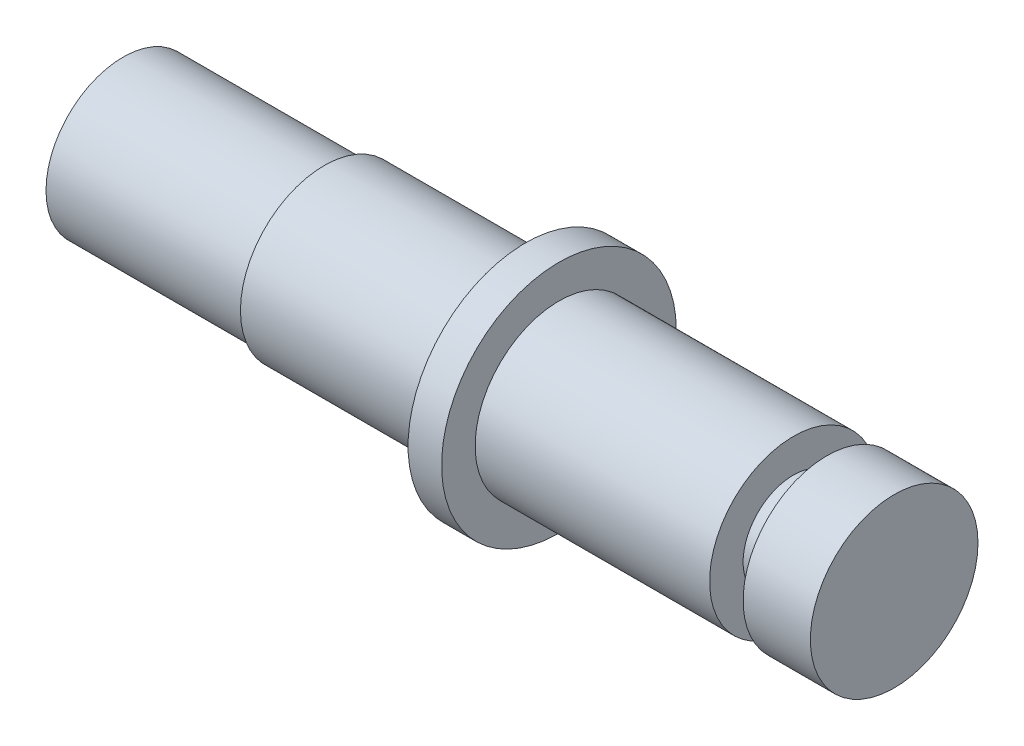
SolidWorks part; units mm, degrees
ref_plane "Front Plane" through (0, 0, 0) normal (0, 0, 1) x (1, 0, 0)
ref_plane "Top Plane" through (0, 0, 0) normal (0, 1, 0) x (1, 0, 0)
ref_plane "Right Plane" through (0, 0, 0) normal (1, 0, 0) x (0, 0, -1)
other "Configuration Table"
sketch "Sketch1" plane through (0, 0, 0) normal (1, 0, 0) x (0, 0, -1)
  circle A0 centre (0, 0) radius 2.3
extrude "Boss-Extrude1" add sketch "Sketch1" along normal blind 20
sketch "Sketch3" plane through (0, 0, 0) normal (0, 0, 1) x (1, 0, 0)
  line L0 (0, 2.3) -> (10, 2.3) construction
  line L1 (20, 2.3) -> (0, 2.3) construction
  line L2 (10, 2.3) -> (10, 2.5)
  line L3 (10, 2.5) -> (10.6945, 2.5)
  line L4 (10.6945, 2.5) -> (10.6945, 2.3)
  line L5 (10.6945, 2.3) -> (10, 2.3)
  line L6 (10, 2.3) -> (10, 0) construction
  line L7 (10, 0) -> (10.6945, 0)
revolve "Revolve1" add sketch "Sketch3" angle 360 about axis through (20, 0, 0) along (-1, 0, 0)
sketch "Sketch4" plane through (0, 0, 0) normal (-1, 0, 0) x (0, 0, 1)
  circle A0 centre (0, 0) radius 2.3
extrude "Boss-Extrude2" add sketch "Sketch4" along normal blind 2
sketch "Sketch5" plane through (20, 0, 0) normal (1, 0, 0) x (0, 0, -1)
  circle A0 centre (0, 0) radius 2.5
extrude "Boss-Extrude3" add sketch "Sketch5" against normal blind 10
sketch "Sketch6" plane through (0.9939, 0, 0) normal (0, 0, 1) x (1, 0, 0)
  line L0 (20, 2.5) -> (18, 2.5) construction
  line L2 (18, 2.5) -> (18, 1.4999)
  line L3 (18, 1.4999) -> (17, 1.4999)
  line L4 (17, 1.4999) -> (17, 2.5)
  line L5 (17, 2.5) -> (18, 2.5)
  line L6 (20, 0) -> (16.6857, 0) construction
revolve "Cut-Revolve1" cut sketch "Sketch6" angle 360 about L6
sketch "Sketch8" plane through (-2, 0, 0) normal (-1, 0, 0) x (0, 0, 1)
  line L0 (0, 0) -> (0, 2.3) construction
  circle A0 centre (0, 0) radius 2.3 construction
ref_plane "Plane1" through (0, 0, 0) normal (0, 0, 1) x (0, 1, 0)
sketch "Sketch9" plane through (0, 0, 0) normal (0, 0, 1) x (0, 1, 0)
  line L0 (1.5, 2) -> (2.3, -4.25) construction
  line L1 (0, 2) -> (2.3, 2) construction
  line L2 (2.3, -10) -> (2.3, 2) construction
  line L3 (2.3, -4.25) -> (0.75, -4.25)
  line L4 (0.75, -4.25) -> (0.75, -4.9347)
  line L5 (0.75, -4.9347) -> (2.3, -4.9347)
  line L6 (2.3, -4.9347) -> (2.3, -4.25)
  line L7 (0, 2) -> (0, -4.6531) construction
  line L8 (2.3, 2) -> (-2.3, 2) construction
  line L9 (-2.3, -4.25) -> (-0.75, -4.25)
  line L10 (-2.3, -4.9347) -> (-2.3, -4.25)
  line L11 (-0.75, -4.9347) -> (-2.3, -4.9347)
  line L12 (-0.75, -4.25) -> (-0.75, -4.9347)
sketch "Sketch10" plane through (10, 0, 0) normal (-1, 0, 0) x (0, 0, 1)
  circle A0 centre (0, 0) radius 2.5
extrude "Boss-Extrude4" add sketch "Sketch10" along normal blind 6
sketch "Sketch11" plane through (0, 0, 0) normal (0, 0, 1) x (1, 0, 0)
  line L0 (4, 2.5) -> (10, 2.5) construction
  line L1 (17.9939, 2.5) -> (4, 2.5) construction
  line L2 (20, 0) -> (5, 0) construction
  line L3 (10, 2.5) -> (11, 2.5)
  line L4 (10, 2.5) -> (10, 3.5)
  line L5 (10, 3.5) -> (11, 3.5)
  line L6 (11, 2.5) -> (11, 3.5)
  line L7 (20, -2.5) -> (20, 2.5) construction
revolve "Revolve2" add sketch "Sketch11" angle 360 about L2
sketch "Sketch12" plane through (20, 0, 0) normal (1, 0, 0) x (0, 0, -1)
  circle A0 centre (0, 0) radius 2.5
extrude "Boss-Extrude5" add sketch "Sketch12" along normal blind 1
